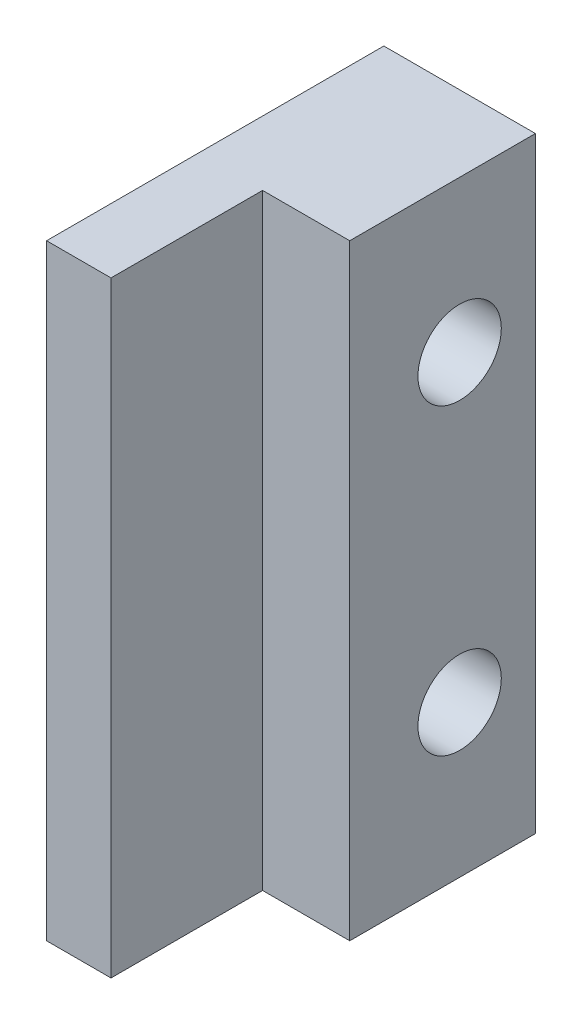
from build123d import *

# Parameters (mm, degrees)
SKETCH_1_3_W        = 20
SKETCH_1_3_H        = 80
BOSS_EXTRUDE1_DEPTH = 8.5
SKETCH_1_3_2_W      = 24.5
SKETCH_1_3_2_H      = 80
SKETCH_1_3_2_R      = 5.5
BOSS_EXTRUDE2_DEPTH = 20


with BuildPart() as part:
    # Sketch 1_3 → Boss-Extrude1 (new body)
    with BuildSketch(Plane(origin=(0, 0, 0), x_dir=(0, 0, -1), z_dir=(1, 0, 0))):
        with Locations((-12.25, 0)):
            Rectangle(SKETCH_1_3_W, SKETCH_1_3_H)
    extrude(amount=BOSS_EXTRUDE1_DEPTH)

    # Sketch 1_3 2 → Boss-Extrude2 (add)
    with BuildSketch(Plane(origin=(0, 0, 0), x_dir=(0, 0, -1), z_dir=(1, 0, 0))):
        with Locations((10, 0)):
            Rectangle(SKETCH_1_3_2_W, SKETCH_1_3_2_H)
        with Locations((12.25, -20)):
            Circle(SKETCH_1_3_2_R, mode=Mode.SUBTRACT)
        with Locations((12.25, 20)):
            Circle(SKETCH_1_3_2_R, mode=Mode.SUBTRACT)
    extrude(amount=BOSS_EXTRUDE2_DEPTH)


solid = part.part
